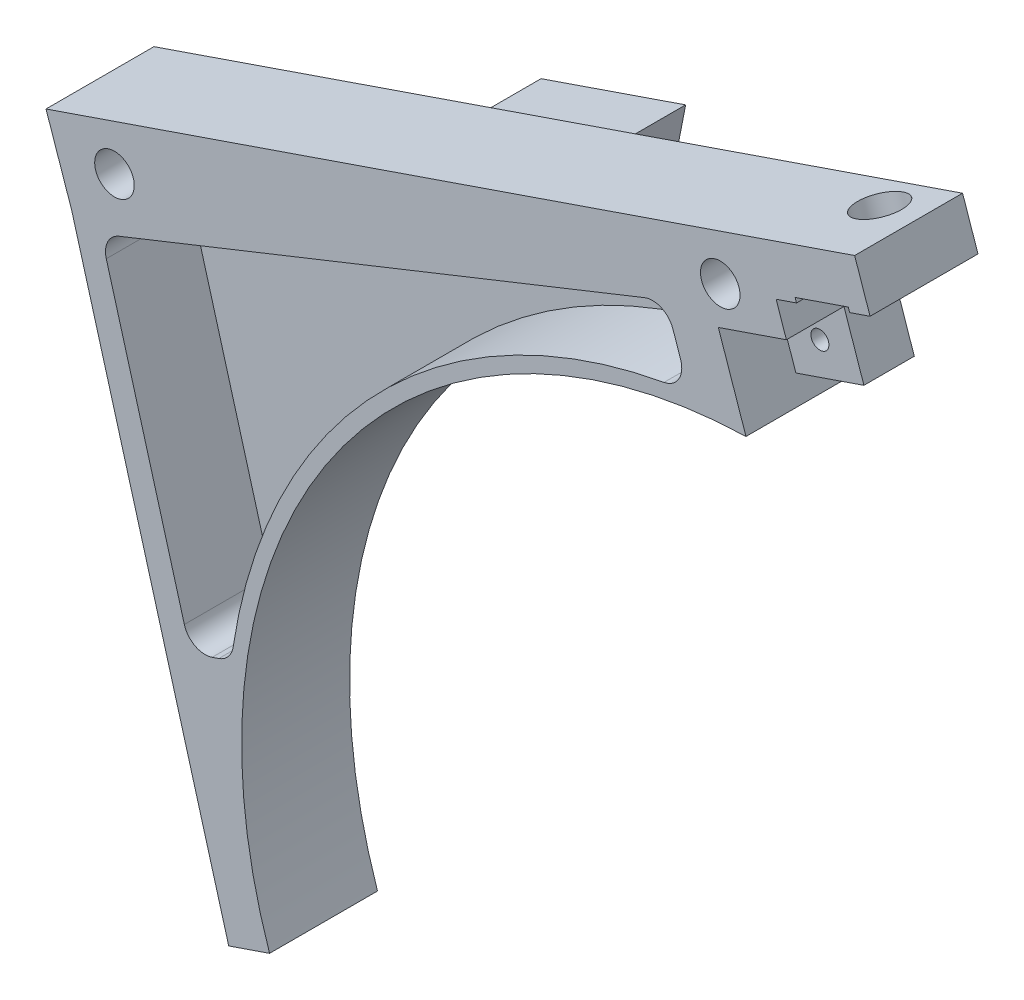
from build123d import *

# Parameters (mm, degrees)
EXTRUDE_1_DEPTH       = 15
EXTRUDE_2_DEPTH       = 8
CUT_EXTRUDE_1_DEPTH   = 12
CUT_EXTRUDE_2_DEPTH   = 8
SKETCH_5_R            = 0.5
CUT_EXTRUDE_3_DEPTH   = 317.640652423
SKETCH_6_R            = 2.75
CUT_EXTRUDE_4_DEPTH   = 317.640652423
HOLE_WIZARD_3_0_3_1_D = 6.5
HOLE_WIZARD_M3_1_D    = 2.5


with BuildPart() as part:
    # 草图1 → 凸台-拉伸1 (new body)
    with BuildSketch(Plane.XY):
        with BuildLine():
            Line((154.501486248, 74.365814355), (160.177770707, 76.310041404))
            ThreePointArc((160.177770707, 76.310041404), (169.160526734, 140.718106761), (226.383321785, 171.615364171))
            Line((226.383321785, 171.615364171), (225.315728088, 174.727294301))
            Line((225.315728088, 174.727294301), (234.77220836, 177.96630476))
            Line((234.77220836, 177.96630476), (231.998602564, 186.064008926))
            Line((231.998602564, 186.064008926), (230.57080221, 190.225905867))
            Line((230.57080221, 190.225905867), (233.408459215, 191.199406109))
            Line((233.408459215, 191.199406109), (233.213759167, 191.76693751))
            Line((233.213759167, 191.76693751), (240.591667381, 194.298038138))
            Line((240.591667381, 194.298038138), (240.786367429, 193.730506737))
            Line((240.786367429, 193.730506737), (243.624024434, 194.704006979))
            Line((243.624024434, 194.704006979), (241.482323903, 200.94685239))
            Line((241.482323903, 200.94685239), (129.111106493, 162.396242824))
            Line((129.111106493, 162.396242824), (132.680607379, 151.991500471))
            Line((132.680607379, 151.991500471), (154.501486248, 74.365814355))
        make_face()
    extrude(amount=EXTRUDE_1_DEPTH)

    # 草图2 → 凸台-拉伸2 (add)
    with BuildSketch(Plane(origin=(0, 0, 0), x_dir=(-1, 0, 0), z_dir=(0, 0, -1))):
        Polygon((-174.908927271, 177.441379972), (-194.997272817, 184.33298428), (-193.224414699, 175.267097261), (-181.873786677, 171.373096295), align=None)
    extrude(amount=EXTRUDE_2_DEPTH)

    # 草图3 → 切除-拉伸1 (cut)
    with BuildSketch(Plane.XY.offset(15)):
        with BuildLine():
            Line((148.33581351, 109.973924886), (137.488957816, 148.560574876))
            ThreePointArc((137.488957816, 148.560574876), (137.68708728, 150.700674405), (139.265834382, 152.159042969))
            Line((139.265834382, 152.159042969), (212.284799547, 181.275892717))
            ThreePointArc((212.284799547, 181.275892717), (214.647795853, 181.215617846), (216.233642795, 179.462770427))
            Line((216.233642795, 179.462770427), (217.297595906, 176.361452247))
            ThreePointArc((217.297595906, 176.361452247), (217.048600661, 173.871762608), (214.998888251, 172.436760111))
            ThreePointArc((214.998888251, 172.436760111), (175.157111586, 151.143900213), (155.117593814, 110.657226135))
            ThreePointArc((155.117593814, 110.657226135), (154.455434588, 109.182984766), (153.12452466, 108.266185323))
            Line((153.12452466, 108.266185323), (152.197376559, 107.948113442))
            ThreePointArc((152.197376559, 107.948113442), (149.830188599, 108.129149559), (148.33581351, 109.973924886))
        make_face()
    extrude(amount=-CUT_EXTRUDE_1_DEPTH, mode=Mode.SUBTRACT)

    # 草图4 → 切除-拉伸2 (cut)
    with BuildSketch(Plane.XY.offset(15)):
        Polygon((234.77220836, 177.96630476), (225.315728088, 174.727294301), (222.53974588, 182.819008121), (231.998602564, 186.064008926), align=None)
    extrude(amount=-CUT_EXTRUDE_2_DEPTH, mode=Mode.SUBTRACT)

    # 草图5 → 切除-拉伸3 (cut, through all)
    with BuildSketch(Plane.XY.offset(15)):
        with Locations((228.656571223, 180.394154027)):
            Circle(SKETCH_5_R)
    extrude(amount=-CUT_EXTRUDE_3_DEPTH, mode=Mode.SUBTRACT)

    # 草图6 → 切除-拉伸4 (cut, through all)
    with BuildSketch(Plane.XY.offset(15)):
        with Locations((138.625192324, 159.316929458)):
            Circle(SKETCH_6_R)
        with Locations((222.809016814, 188.197436624)):
            Circle(SKETCH_6_R)
    extrude(amount=-CUT_EXTRUDE_4_DEPTH, mode=Mode.SUBTRACT)

    # Ø3.0 (3) 直径孔1 (through all)
    with Locations(Plane(origin=(-34.303459783, 99.991195485, 0), x_dir=(-0.9458856684292948, -0.32450008052397505, 0), z_dir=(0.32450008052397505, -0.9458856684292948, 0))):
        with Locations((-286.72193914, -5)):
            Hole(HOLE_WIZARD_3_0_3_1_D / 2)

    # M3 螺纹孔1 (through all)
    with Locations(Plane.XY.offset(7)):
        with Locations((228.656571223, 180.394154027)):
            Hole(HOLE_WIZARD_M3_1_D / 2)


solid = part.part
